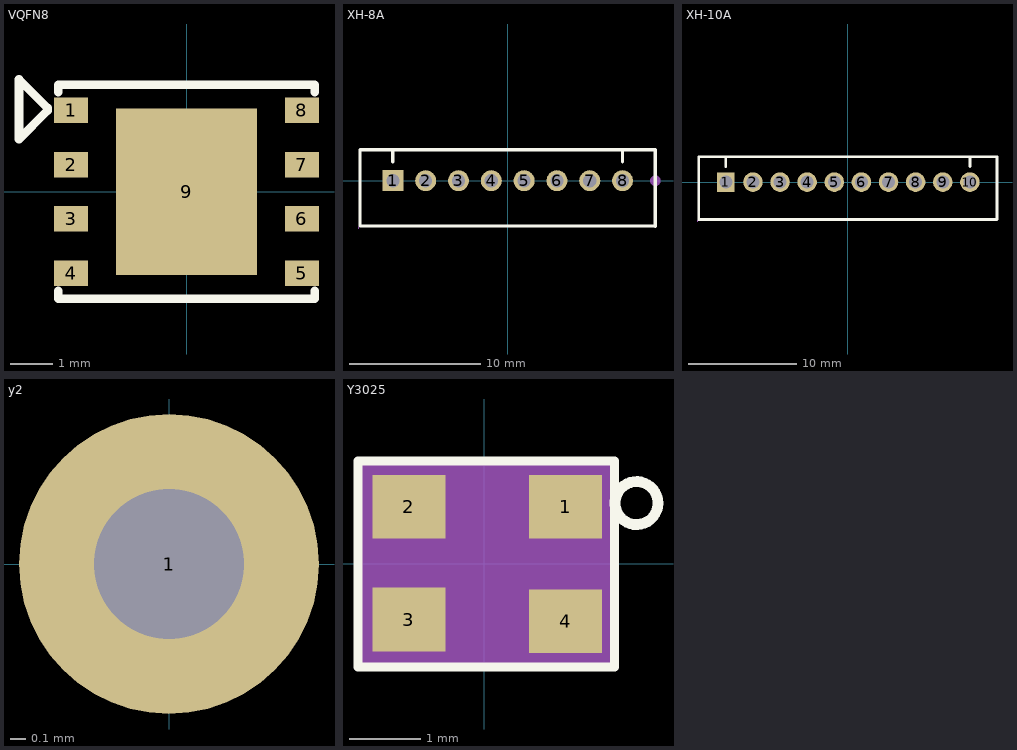
[diagram p0: the footprints below, top view; thin cyan lines are the x and y axes]
# Altium footprint library MISC84456-5.PcbLib: 85 footprints (part 6 of 6)
Each footprint in its own frame and in the unit in brackets; x right, y up, seen from the top. Pads: shape width x height; smd on the part's side, far side on the other; paste and mask are expansions set on the pad; w line width, h text height; cw(c..) or ccw(c..) is an arc to the next point about the centre after c.

## VQFN8 [mm]
pads (9):
  rect 0.8x0.6 smd: 1(-2.7,1.905) 2(-2.7,0.635) 3(-2.7,-0.635) 4(-2.7,-1.905) 5(2.7,-1.905) 6(2.7,-0.635) 7(2.7,0.635) 8(2.7,1.905)
  rect 3.3x3.9 smd: 9(0,0)
Top Overlay:
  lines w0.2: -3.25,1.95 -3.25,1.96 ; -3,-2.32 -3,-2.5 3,-2.5 3,-2.32 ; -3,2.33 -3,2.5 3,2.5 3,2.33 ; -3.25,1.96 -3.92,2.63 -3.92,1.23 -3.25,1.9 -3.25,1.96

## XH-8A [mm]
pads (8):
  rect 1.6x1.6 hole 1: 1(-8.75,0)
  round 1.6 hole 1: 2(-6.25,0) 3(-3.75,0) 4(-1.25,0) 5(1.25,0) 6(3.75,0) 7(6.25,0) 8(8.75,0)
Top Overlay:
  lines w0.254: -8.75,1.45 -8.75,2.35 ; 8.74,1.44 8.74,2.339 ; 11.24,-3.46 11.24,2.34 ; 11.25,-3.45 -11.25,-3.45 -11.25,2.35 11.25,2.35
Mechanical 5:
  circle w0.4: c11.25,0 r0.2
  circle w0.4: c8.75,0 r0.2
  circle w0.4: c6.25,0 r0.2
  circle w0.4: c3.75,0 r0.2
  circle w0.4: c1.25,0 r0.2
  circle w0.4: c-1.25,0 r0.2
  circle w0.4: c-3.75,0 r0.2
  circle w0.4: c-6.25,0 r0.2
  circle w0.4: c-8.75,0 r0.2
Mechanical 6:
  circle w0.06: c-11.377,-3.577 r0.03

## XH-10A [mm]
pads (10):
  rect 1.6x1.8 hole 1.2: 1(-11.25,0)
  round 1.8 hole 1.2: 2(-8.75,0) 3(-6.25,0) 4(-3.75,0) 5(-1.25,0) 6(1.25,0) 7(3.75,0) 8(6.25,0) 9(8.75,0) 10(11.25,0)
Top Overlay:
  lines w0.254: -11.25,1.45 -11.25,2.35 ; 11.25,1.45 11.25,2.35 ; -13.75,-3.45 13.75,-3.45 13.75,2.35 -13.75,2.35 -13.75,-3.45
Mechanical 5:
  circle w0.5: c-11.25,0 r0.25
  circle w0.5: c-8.75,0 r0.25
  circle w0.5: c-6.25,0 r0.25
  circle w0.5: c-3.75,0 r0.25
  circle w0.5: c-1.25,0 r0.25
  circle w0.5: c1.25,0 r0.25
  circle w0.5: c3.75,0 r0.25
  circle w0.5: c6.25,0 r0.25
  circle w0.5: c8.75,0 r0.25
  circle w0.5: c11.25,0 r0.25
Mechanical 6:
  circle w0.06: c-13.877,-3.577 r0.03

## y2 [mm]
pads (1):
  round 2 hole 1 unplated: 1(0,0)

## Y3025 [mil] "Y3025"
pads (4):
  rect 40x35 smd: 1(44.66,31.5) 2(-41.34,31.5) 3(-41.34,-30.5) 4(44.66,-31.5)
Top Overlay:
  circle w5.91: c83.66,33.46 r11.81
  lines w5: -69.34,-56.5 -69.34,41.5 -69.34,56.5 71.66,56.5 71.66,-56.5 -69.34,-56.5
Mechanical 7:
  text "4" at 42.26,-31.5 h3
  text "2" at -43.74,31.5 h3
  text "3" at -43.74,-30.5 h3
  text "1" at 42.26,31.5 h3
Mechanical 8:
  region: -68.9,55.12 -68.9,-55.12 68.9,-55.12 68.9,55.12
Mechanical 9:
  text "12Mhz20pF" at -58.07,-8.86 h13.78
  text ".Designator" at -19.69,-6.89 h13.78